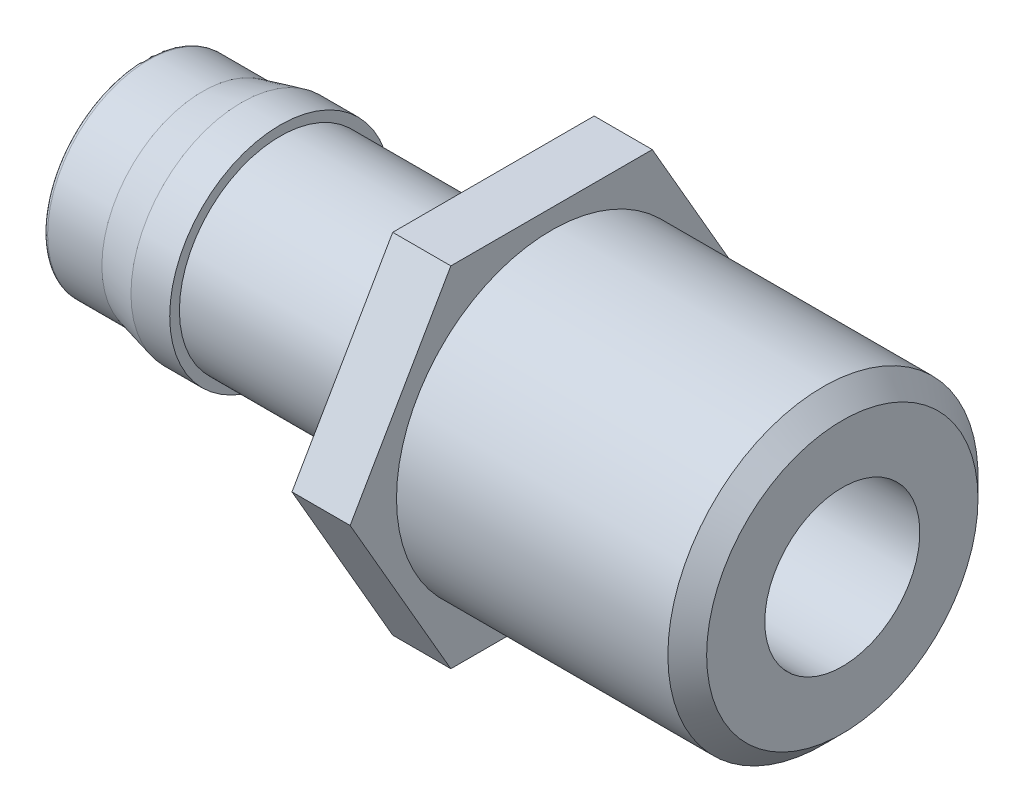
SolidWorks part; units mm, degrees
material "H62"
ref_plane "Front Plane" through (0, 0, 0) normal (0, 0, 1) x (1, 0, 0)
ref_plane "Top Plane" through (0, 0, 0) normal (0, 1, 0) x (1, 0, 0)
ref_plane "Right Plane" through (0, 0, 0) normal (1, 0, 0) x (0, 0, -1)
sketch "Sketch1" plane through (0, 0, 0) normal (0, 0, 1) x (1, 0, 0)
  line L0 (0, 0) -> (22.0497, 0) construction
  line L1 (0, 2) -> (18, 2)
  line L2 (0, 2) -> (0, 2.6)
  line L3 (0, 2.6) -> (1.5, 2.6)
  line L4 (1.5, 2.6) -> (2.5, 2.85)
  line L5 (2.5, 2.85) -> (3.5, 2.85)
  line L6 (3.5, 2.85) -> (3.5, 2.6)
  line L7 (3.5, 2.6) -> (9, 2.6)
  line L8 (9, 2.6) -> (9, 6)
  line L9 (9, 6) -> (10.5, 6)
  line L10 (10.5, 6) -> (10.5, 4)
  line L11 (10.5, 4) -> (18, 4)
  line L12 (18, 4) -> (18, 2)
  dimension "D1" = 18
  dimension "D2" = 1.5
  dimension "D3" = 1
  dimension "D4" = 4
  dimension "D5" = 5.2
  dimension "D6" = 5.7
  dimension "D7" = 5.2
  dimension "D8" = 12
  dimension "D9" = 8
  dimension "D10" = 5.5
  dimension "D11" = 7.5
  dimension "D12" = 9
revolve "Revolve1" add sketch "Sketch1" angle 360 about L0
cosmetic thread "Cosmetic Thread1" parameters "D1"=7.5, "D2"=6.647
sketch "Sketch2" plane through (10.5, 0, 0) normal (1, 0, 0) x (0, 0, -1)
  line L1 (2.5981, -4.5) -> (5.1962, 0)
  line L2 (5.1962, 0) -> (2.5981, 4.5)
  line L3 (2.5981, 4.5) -> (-2.5981, 4.5)
  line L4 (-2.5981, 4.5) -> (-5.1962, 0)
  line L5 (-5.1962, 0) -> (-2.5981, -4.5)
  line L6 (-2.5981, -4.5) -> (2.5981, -4.5)
  circle A0 centre (0, 0) radius 4.5 construction
  dimension "D1" = 9
extrude "Cut-Extrude3" cut sketch "Sketch2" against normal blind 10 flip side to cut
fillet "Fillet1" radius 0.1 1 edges at (0, 0, 2.6)
chamfer "Chamfer1" distance 0.5 angle 45 1 edges at (18, 0, 4)
